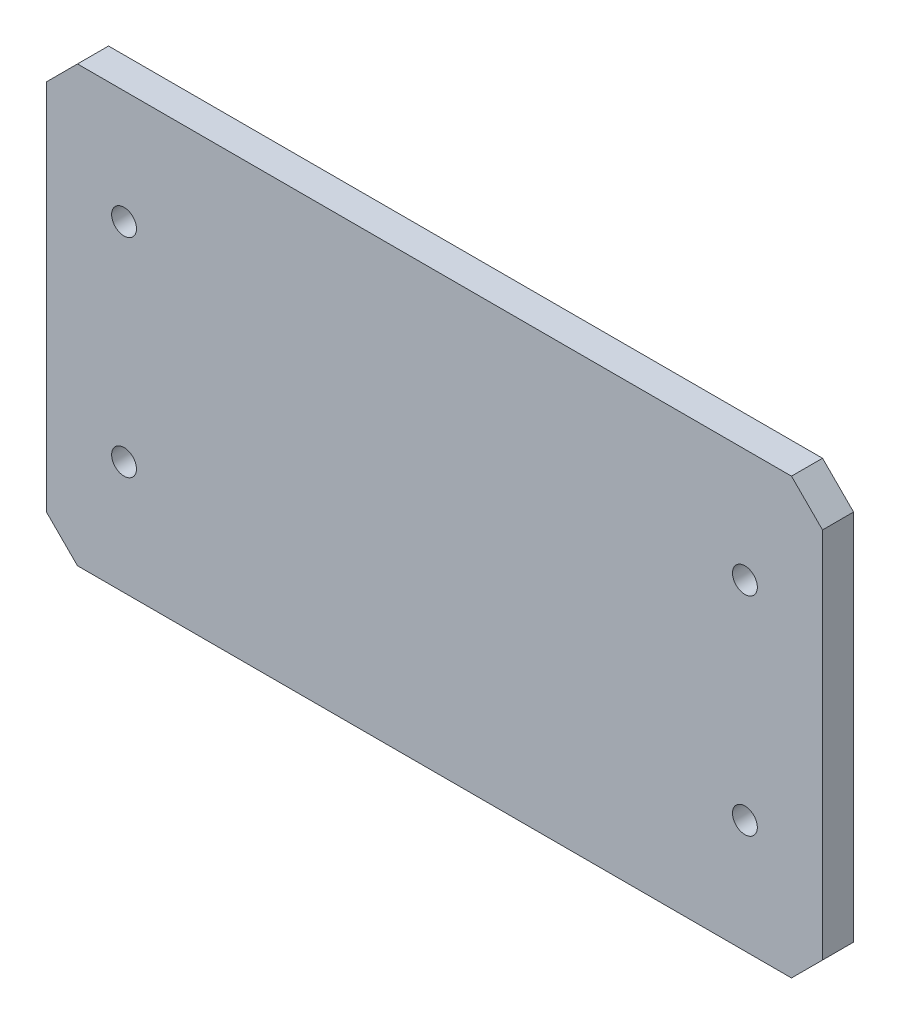
from build123d import *

# Parameters (mm, degrees)
BOSS_EXTRUDE1_DEPTH = 10
SKETCH6_R           = 4
CUT_EXTRUDE3_DEPTH  = 5
BOSS_EXTRUDE3_START = 5
SKETCH7_R           = 4
BOSS_EXTRUDE3_DEPTH = 5
SKETCH8_R           = 4
CUT_EXTRUDE4_DEPTH  = 5
SKETCH11_R          = 4
CUT_EXTRUDE5_DEPTH  = 10


with BuildPart() as part:
    # Sketch1 → Boss-Extrude1 (new body)
    with BuildSketch(Plane.XY):
        Polygon((-115, 70), (-125, 60), (-125, -60), (-115, -70), (115, -70), (125, -60), (125, 60), (115, 70), align=None)
    extrude(amount=BOSS_EXTRUDE1_DEPTH)

    # Sketch6 → Cut-Extrude3 (cut)
    with BuildSketch(Plane(origin=(0, 0, 0), x_dir=(-1, 0, 0), z_dir=(0, 0, -1))):
        with Locations((79.1, 0)):
            Circle(SKETCH6_R)
        with Locations(Location((-79.1, 0, 0), (0, 0, 180))):
            Circle(SKETCH6_R)
    extrude(amount=-CUT_EXTRUDE3_DEPTH, mode=Mode.SUBTRACT)

    # Sketch7 → Boss-Extrude3 (add)
    with BuildSketch(Plane(origin=(0, 0, 5), x_dir=(-1, 0, 0), z_dir=(0, 0, -1)).offset(BOSS_EXTRUDE3_START)):
        with Locations((79.1, 0)):
            Circle(SKETCH7_R)
    extrude(amount=-BOSS_EXTRUDE3_DEPTH)

    # Sketch8 → Cut-Extrude4 (cut)
    with BuildSketch(Plane(origin=(0, 0, 0), x_dir=(-1, 0, 0), z_dir=(0, 0, -1))):
        with Locations((-50, -64.1)):
            Circle(SKETCH8_R)
        with Locations(Location((50, -64.1, 0), (0, 0, 180))):
            Circle(SKETCH8_R)
    extrude(amount=-CUT_EXTRUDE4_DEPTH, mode=Mode.SUBTRACT)

    # Sketch11 → Cut-Extrude5 (cut)
    with BuildSketch(Plane.XY.offset(10)):
        with Locations((100, 33.5)):
            Circle(SKETCH11_R)
        with Locations(Location((-100, 33.5, 0), (0, 0, 180))):
            Circle(SKETCH11_R)
        with Locations((-100, -33.5)):
            Circle(SKETCH11_R)
        with Locations(Location((100, -33.5, 0), (0, 0, 180))):
            Circle(SKETCH11_R)
    extrude(amount=-CUT_EXTRUDE5_DEPTH, mode=Mode.SUBTRACT)


solid = part.part
